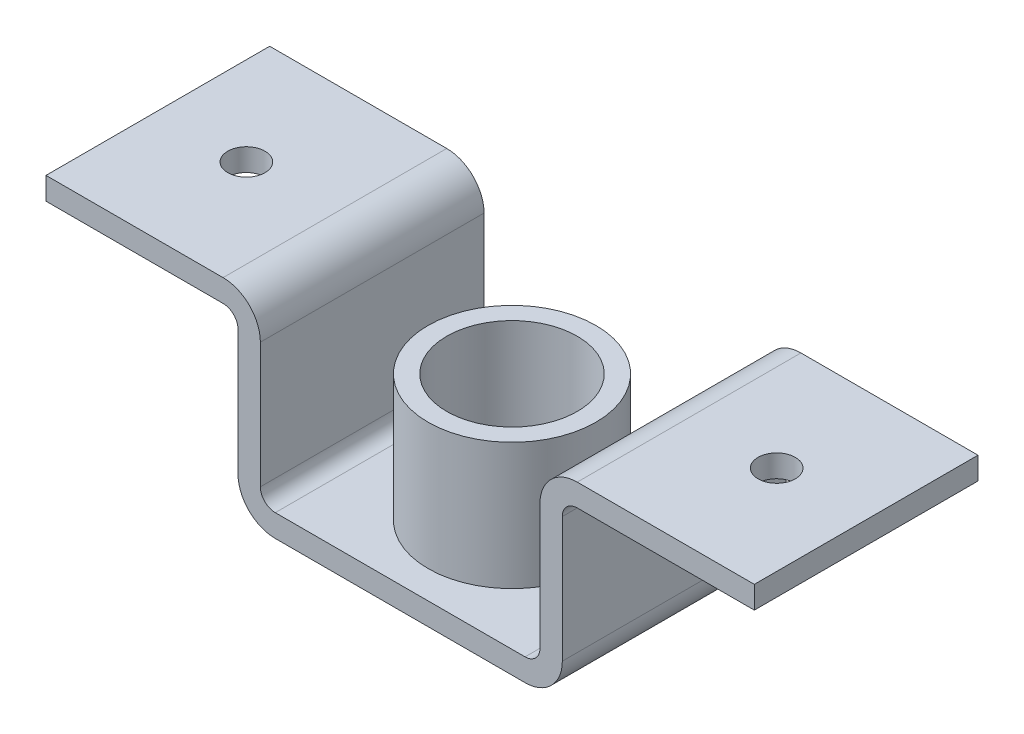
SolidWorks part; units mm, degrees
ref_plane "Front Plane" through (0, 0, 0) normal (0, 0, 1) x (1, 0, 0)
ref_plane "Top Plane" through (0, 0, 0) normal (0, 1, 0) x (1, 0, 0)
ref_plane "Right Plane" through (0, 0, 0) normal (1, 0, 0) x (0, 0, -1)
sketch "Sketch1" plane through (0, 0, 0) normal (0, 0, 1) x (1, 0, 0)
  line L0 (187.5, 0) -> (-187.5, 0)
  line L1 (-187.5, 0) -> (-187.5, 238)
  line L2 (-187.5, 238) -> (-475, 238)
  line L3 (0, 487.8375) -> (0, -366.993) construction
  line L4 (-475, 238) -> (-475, 208)
  line L5 (-475, 208) -> (-217.5, 208)
  line L6 (-217.5, 208) -> (-217.5, -30)
  line L7 (-217.5, -30) -> (217.5, -30)
  line L8 (217.5, 208) -> (217.5, -30)
  line L9 (475, 208) -> (217.5, 208)
  line L10 (475, 238) -> (475, 208)
  line L11 (187.5, 238) -> (475, 238)
  line L12 (187.5, 0) -> (187.5, 238)
  point P12 (0, -30)
  point P17 (0, 0)
  dimension "D1" = 187.5
  dimension "D2" = 475
  dimension "D3" = 238
  dimension "D4" = 30
  dimension "D5" = 30
  dimension "D6" = 30
extrude "Boss-Extrude2" add sketch "Sketch1" along normal blind 300
fillet "Fillet3" radius 20 2 edges at (187.5, 0, 150) (-187.5, 0, 150)
fillet "Fillet4" radius 50 4 edges at (217.5, -30, 150) (-217.5, -30, 150) (187.5, 238, 150) (-187.5, 238, 150)
fillet "Fillet5" radius 20 2 edges at (-217.5, 208, 150) (217.5, 208, 150)
sketch "Sketch2" plane through (0, 0, 0) normal (0, 1, 0) x (1, 0, 0)
  line L0 (0, 90.4266) -> (0, -300) construction
  line L1 (167.5, -300) -> (-167.5, -300) construction
  line L2 (167.5, 0) -> (-167.5, 0) construction
  circle A0 centre (0, -150) radius 112.5
  circle A1 centre (0, -150) radius 87.5
  dimension "D1" = 225
  dimension "D2" = 175
  dimension "D3" = 150
extrude "Boss-Extrude3" add sketch "Sketch2" along normal blind 170
sketch "Sketch3" plane through (0, 0, 0) normal (0, 1, 0) x (1, 0, 0)
  circle A0 centre (0, -150) radius 37.5
  dimension "D1" = 75
extrude "Cut-Extrude1" cut sketch "Sketch3" against normal up to next
sketch "Sketch4" plane through (0, 238, 0) normal (0, 1, 0) x (1, 0, 0)
  line L0 (-356.25, 0) -> (-356.25, -300) construction
  line L1 (-237.5, 0) -> (-475, 0) construction
  line L2 (-237.5, -300) -> (-475, -300) construction
  line L3 (475, -300) -> (475, 0) construction
  circle A0 centre (-356.25, -150) radius 25
  circle A1 centre (355, -150) radius 25
  point P10 (475, -150)
  dimension "D1" = 50
  dimension "D2" = 120
extrude "Cut-Extrude2" cut sketch "Sketch4" against normal up to next
